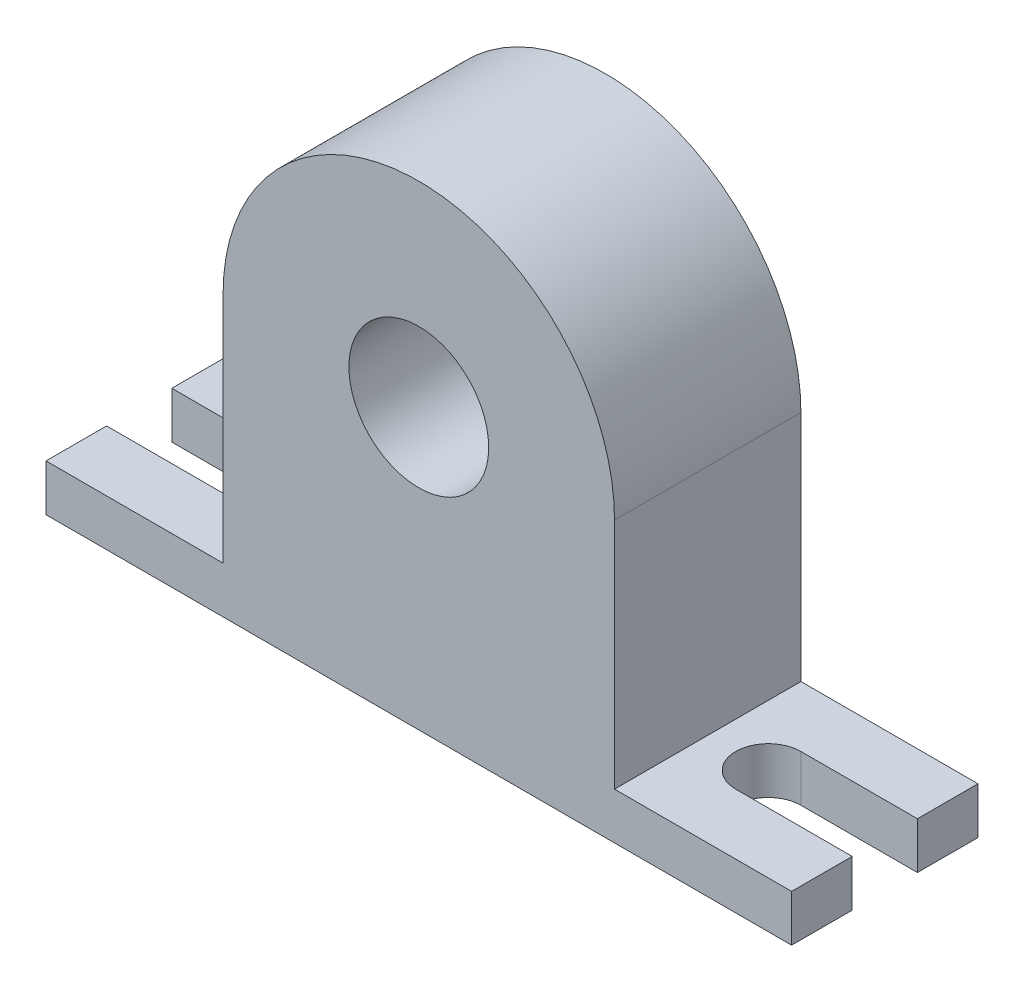
SolidWorks part; units mm, degrees
ref_plane "前视基准面" through (0, 0, 0) normal (0, 0, 1) x (1, 0, 0)
ref_plane "上视基准面" through (0, 0, 0) normal (0, 1, 0) x (1, 0, 0)
ref_plane "右视基准面" through (0, 0, 0) normal (1, 0, 0) x (0, 0, -1)
sketch "草图1" plane through (0, 0, 0) normal (0, 0, 1) x (1, 0, 0)
  line L0 (21, 0) -> (21, -25)
  line L1 (21, -30) -> (40, -30)
  line L2 (40, -30) -> (40, -25)
  line L3 (40, -25) -> (21, -25)
  line L4 (0, 27.0922) -> (0, -50.8158) construction
  line L5 (-21, -30) -> (-40, -30)
  line L6 (-40, -30) -> (-40, -25)
  line L7 (-40, -25) -> (-21, -25)
  line L8 (-21, 0) -> (-21, -25)
  line L9 (-21, -30) -> (21, -30)
  arc A0 (21, 0) -> (-21, 0) centre (0, 0) ccw
  circle A1 centre (0, 0) radius 7.5
  dimension "D1" = 42
  dimension "D5" = 15
  dimension "D2" = 19
  dimension "D3" = 5
  dimension "D4" = 30
extrude "凸台-拉伸1" add sketch "草图1" along normal blind 20
sketch "草图2" plane through (0, -25, 0) normal (0, 1, 0) x (1, 0, 0)
  line L0 (0, 8.4897) -> (0, -30.2387) construction
  line L1 (-27.5, -6.5) -> (-40, -6.5)
  line L2 (-40, -20) -> (-40, 0) construction
  line L3 (-40, -6.5) -> (-40, -13.5)
  line L4 (-40, -13.5) -> (-27.5, -13.5)
  line L5 (40, -13.5) -> (27.5, -13.5)
  line L6 (40, -6.5) -> (40, -13.5)
  line L7 (27.5, -6.5) -> (40, -6.5)
  arc A0 (-27.5, -13.5) -> (-27.5, -6.5) centre (-27.5, -10) ccw
  arc A1 (27.5, -13.5) -> (27.5, -6.5) centre (27.5, -10) cw
  dimension "D2" = 3.5
  dimension "D1" = 27.5
extrude "切除-拉伸1" cut sketch "草图2" against normal through all
